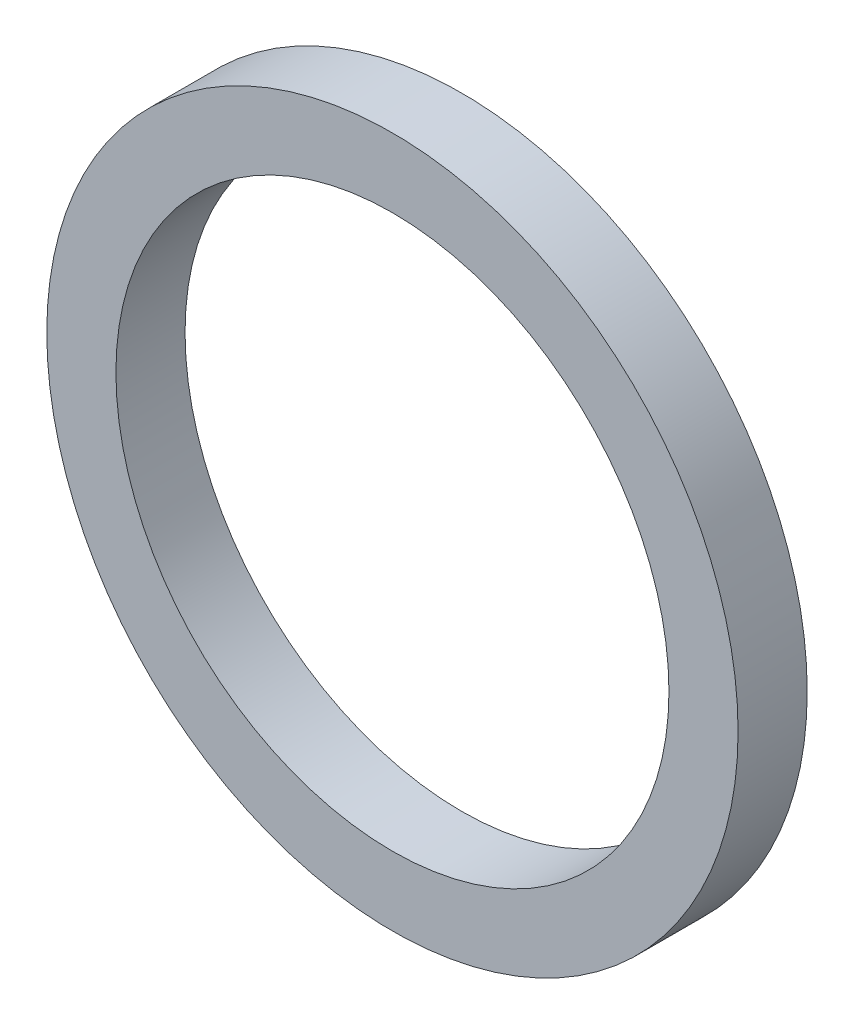
SolidWorks part; units mm, degrees
material "H62"
ref_plane "前视基准面" through (0, 0, 0) normal (0, 0, 1) x (1, 0, 0)
ref_plane "上视基准面" through (0, 0, 0) normal (0, 1, 0) x (1, 0, 0)
ref_plane "右视基准面" through (0, 0, 0) normal (1, 0, 0) x (0, 0, -1)
sketch "草图1" plane through (0, 0, 0) normal (0, 0, 1) x (1, 0, 0)
  circle A0 centre (0, 0) radius 25
  circle A1 centre (0, 0) radius 20
  dimension "D1" = 40
  dimension "D2" = 50
extrude "凸台-拉伸1" add sketch "草图1" along normal blind 5
